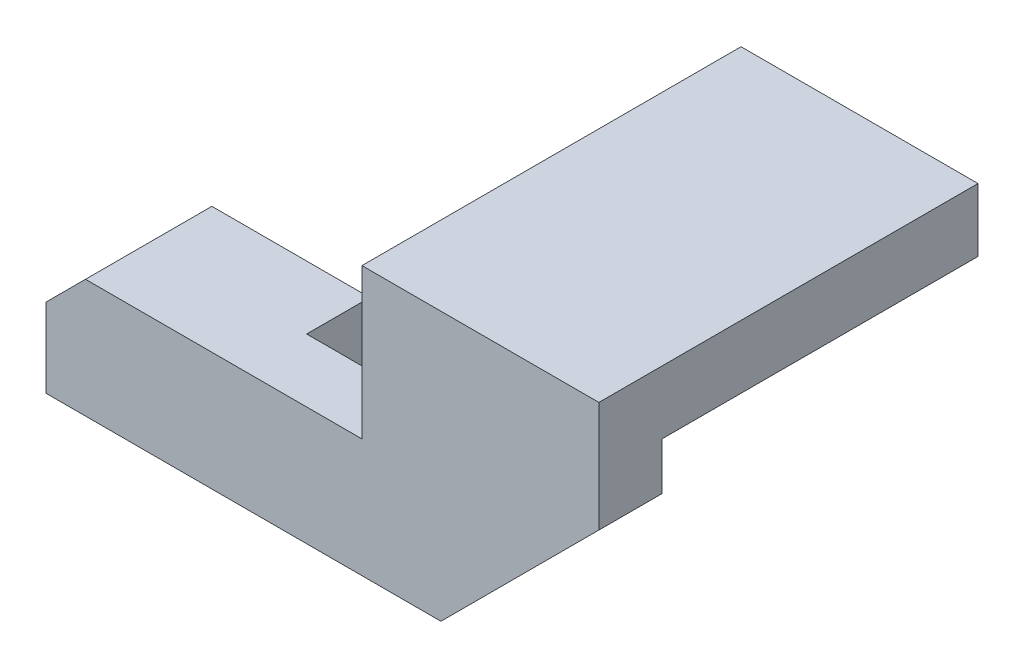
SolidWorks part; units mm, degrees
ref_plane "Front Plane" through (0, 0, 0) normal (0, 0, 1) x (1, 0, 0)
ref_plane "Top Plane" through (0, 0, 0) normal (0, 1, 0) x (1, 0, 0)
ref_plane "Right Plane" through (0, 0, 0) normal (1, 0, 0) x (0, 0, -1)
sketch "Sketch1" plane through (0, 0, 0) normal (0, 1, 0) x (1, 0, 0)
  line L0 (-15, 20) -> (15, -20) construction
  line L1 (-15, 20) -> (15, 20)
  line L2 (-15, 20) -> (-15, -20)
  line L3 (-15, -20) -> (15, -20)
  line L4 (15, 20) -> (15, -20)
  dimension "D1" = 40
  dimension "D2" = 30
extrude "Boss-Extrude1" add sketch "Sketch1" along normal blind 8
sketch "Sketch2" plane through (0, 0, 20) normal (0, 0, 1) x (1, 0, 0)
  line L0 (15, 8) -> (15, 0) construction
  line L1 (-15, 8) -> (15, 8)
  line L2 (-15, 8) -> (-15, -26)
  line L3 (-15, -26) -> (15, -26)
  line L4 (15, 8) -> (15, -26)
  dimension "D1" = 34
extrude "Boss-Extrude2" add sketch "Sketch2" along normal blind 8
sketch "Sketch3" plane through (-15, 0, 0) normal (-1, 0, 0) x (0, 0, 1)
  line L0 (28, 8) -> (28, -26) construction
  line L1 (20, -26) -> (28, -26)
  line L2 (20, -26) -> (20, -11)
  line L3 (20, -11) -> (28, -11)
  line L4 (28, -26) -> (28, -11)
  dimension "D1" = 15
extrude "Boss-Extrude3" add sketch "Sketch3" along normal blind 40
chamfer "Chamfer1" distance 5 angle 45 1 edges at (-55, -11, 24)
sketch "Sketch4" plane through (0, 0, 20) normal (0, 0, -1) x (-1, 0, 0)
  line L0 (30, -11) -> (50, -11)
  line L1 (50, -11) -> (55, -16)
  line L2 (55, -16) -> (55, -26)
  line L3 (55, -26) -> (30, -26)
  line L4 (55, -26) -> (-15, -26) construction
  line L5 (30, -26) -> (30, -11)
  dimension "D1" = 20
extrude "Boss-Extrude4" add sketch "Sketch4" along normal blind 8
chamfer "Chamfer2" distance 20 angle 45 1 edges at (15, -26, 24)
